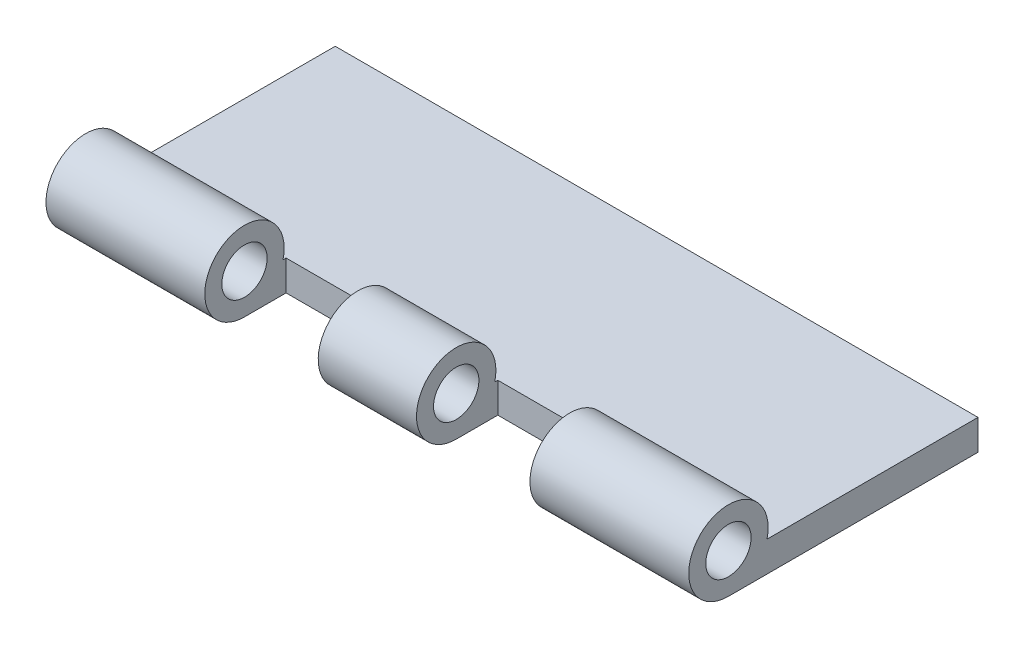
from build123d import *

# Parameters (mm, degrees)
BOSS_EXTRUDE1_DEPTH = 42.5
SKETCH3_W           = 15
SKETCH3_H           = 11
CUT_EXTRUDE2_DEPTH  = 10
SKETCH4_R           = 3
CUT_EXTRUDE3_DEPTH  = 92.332154798


with BuildPart() as part:
    # Sketch1 → Boss-Extrude1 (new, symmetric)
    with BuildSketch(Plane(origin=(0, 0, 0), x_dir=(0, 0, -1), z_dir=(1, 0, 0))):
        with BuildLine():
            Line((5.099019514, -1.25), (33, -1.25))
            Line((33, -1.25), (33, -5.25))
            Line((33, -5.25), (0, -5.25))
            ThreePointArc((0, -5.25), (-3.240370349, 4.13067791), (5.099019514, -1.25))
        make_face()
    extrude(amount=BOSS_EXTRUDE1_DEPTH, both=True)

    # Sketch3 → Cut-Extrude2 (cut, symmetric)
    with BuildSketch(Plane(origin=(0, 0, 0), x_dir=(1, 0, 0), z_dir=(0, 1, 0))):
        with Locations((14, 0)):
            Rectangle(SKETCH3_W, SKETCH3_H)
        with Locations((-14, 0)):
            Rectangle(SKETCH3_W, SKETCH3_H)
    extrude(amount=CUT_EXTRUDE2_DEPTH, both=True, mode=Mode.SUBTRACT)

    # Sketch4 → Cut-Extrude3 (cut, through all)
    with BuildSketch(Plane(origin=(42.5, 0, 0), x_dir=(0, 0, -1), z_dir=(1, 0, 0))):
        Circle(SKETCH4_R)
    extrude(amount=-CUT_EXTRUDE3_DEPTH, mode=Mode.SUBTRACT)


solid = part.part
